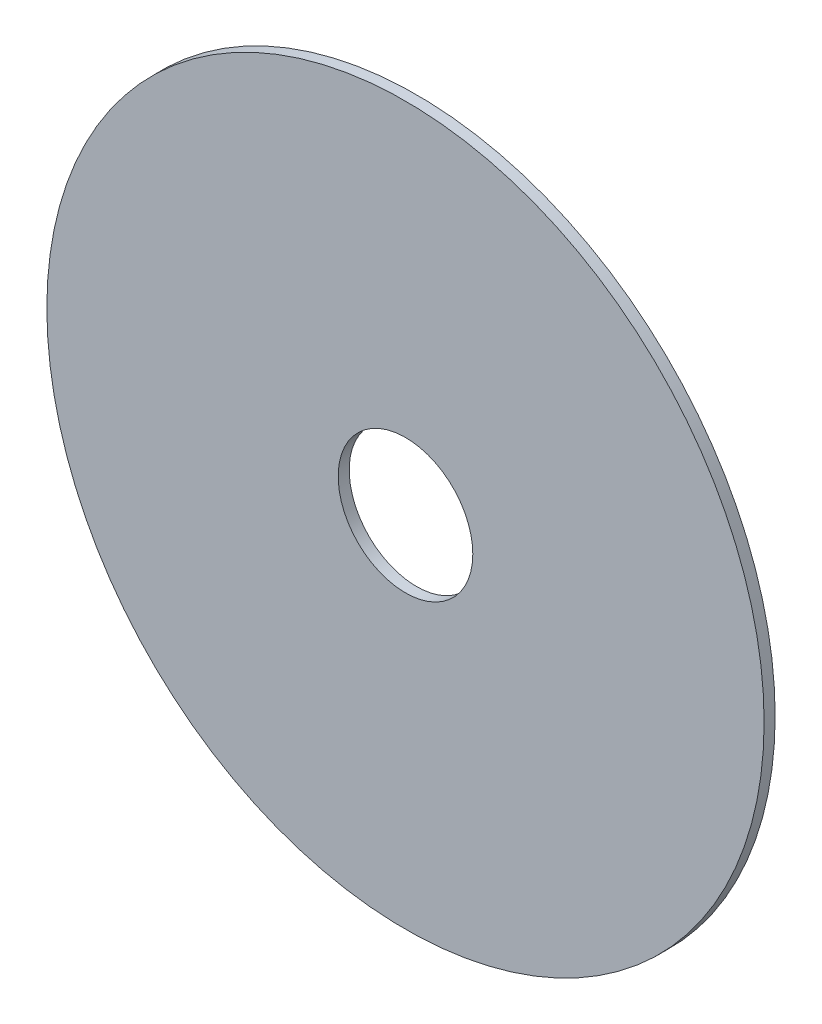
from build123d import *

# Parameters (mm, degrees)
SKETCH1_R           = 162.5
SKETCH1_R_2         = 30.5
BOSS_EXTRUDE1_DEPTH = 5


with BuildPart() as part:
    # Sketch1 → Boss-Extrude1 (new body)
    with BuildSketch(Plane.XY):
        Circle(SKETCH1_R)
        Circle(SKETCH1_R_2, mode=Mode.SUBTRACT)
    extrude(amount=BOSS_EXTRUDE1_DEPTH)


solid = part.part
